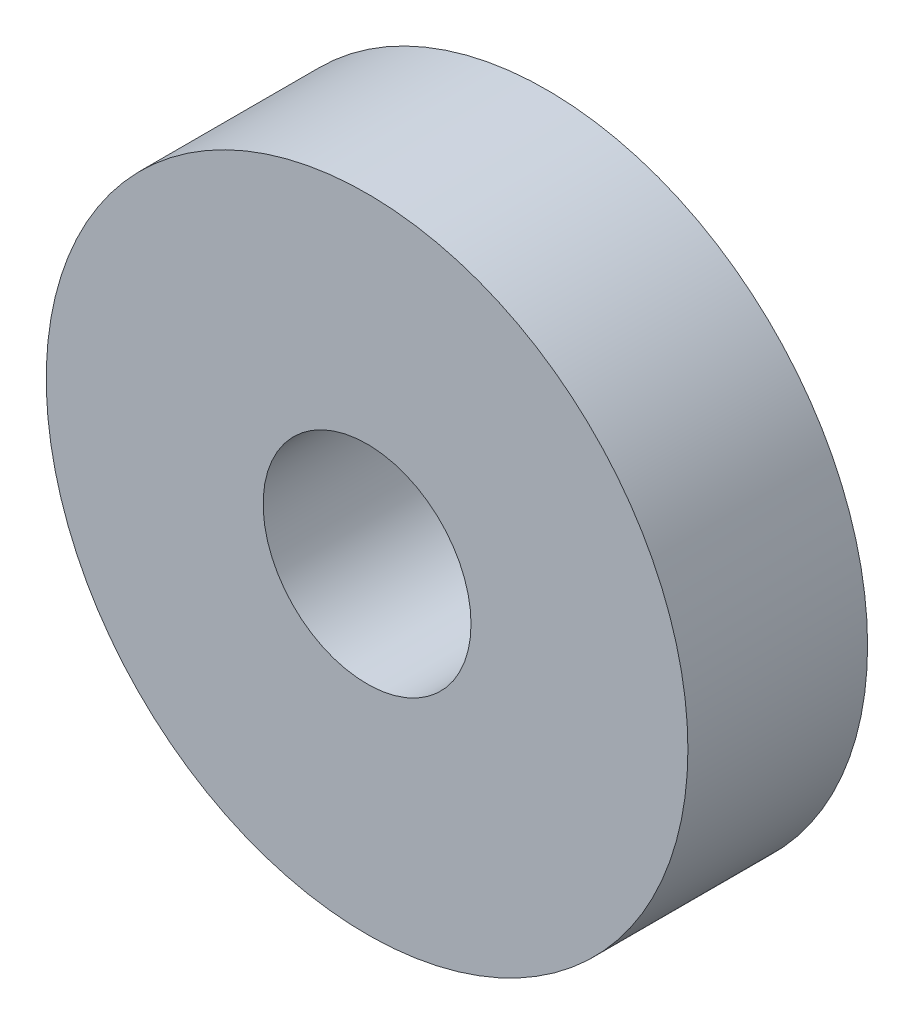
SolidWorks part; units mm, degrees
ref_plane "前视基准面" through (0, 0, 0) normal (0, 0, 1) x (1, 0, 0)
ref_plane "上视基准面" through (0, 0, 0) normal (0, 1, 0) x (1, 0, 0)
ref_plane "右视基准面" through (0, 0, 0) normal (1, 0, 0) x (0, 0, -1)
other "Configuration Table"
sketch "草图1" plane through (0, 0, 0) normal (0, 0, 1) x (1, 0, 0)
  circle A0 centre (0, 0) radius 25
  circle A1 centre (0, 0) radius 8.1
  point P0 (0, 0)
  dimension "D1" = 16.2
  dimension "D2" = 50
extrude "凸台-拉伸1" add sketch "草图1" against normal mid plane 14
